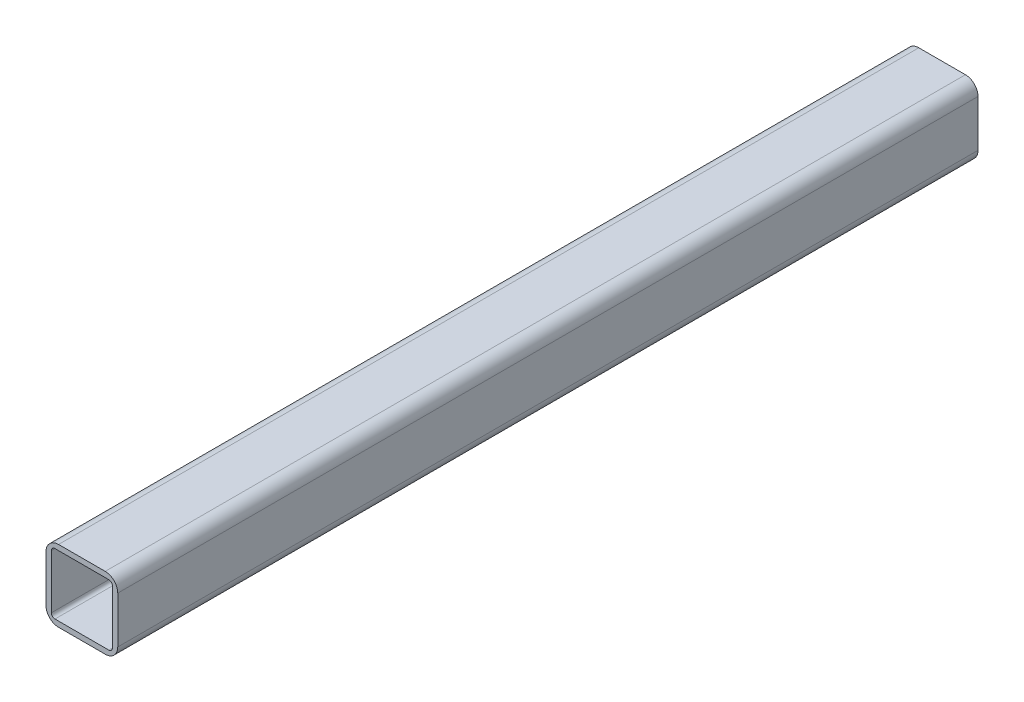
SolidWorks part; units mm, degrees
material "Q235A"
ref_plane "Front Plane" through (0, 0, 0) normal (0, 0, 1) x (1, 0, 0)
ref_plane "Top Plane" through (0, 0, 0) normal (0, 1, 0) x (1, 0, 0)
ref_plane "Right Plane" through (0, 0, 0) normal (1, 0, 0) x (0, 0, -1)
sketch "Sketch1" plane through (0, 0, 0) normal (0, 0, 1) x (1, 0, 0)
  line L1 (-20, 20) -> (20, 20)
  line L2 (-20, 20) -> (-20, -20)
  line L3 (-20, -20) -> (20, -20)
  line L4 (20, 20) -> (20, -20)
  line L5 (-20, 20) -> (20, -20) construction
  line L6 (-20, -20) -> (20, 20) construction
  line L7 (-17, 17) -> (17, 17)
  line L8 (-17, 17) -> (-17, -17)
  line L9 (-17, -17) -> (17, -17)
  line L10 (17, 17) -> (17, -17)
  line L11 (-17, 17) -> (17, -17) construction
  line L12 (-17, -17) -> (17, 17) construction
  point P0 (0, 0)
  point P6 (0, 0)
  dimension "D1" = 40
  dimension "D2" = 40
  dimension "D3" = 3
  dimension "D4" = 3
extrude "Boss-Extrude1" add sketch "Sketch1" along normal blind 479.48
fillet "Fillet1" radius 2 4 edges at (17, 17, 239.74) (-17, 17, 239.74) (-17, -17, 239.74) (17, -17, 239.74)
fillet "Fillet2" radius 7 4 edges at (20, 20, 239.74) (20, -20, 239.74) (-20, 20, 239.74) (-20, -20, 239.74)
